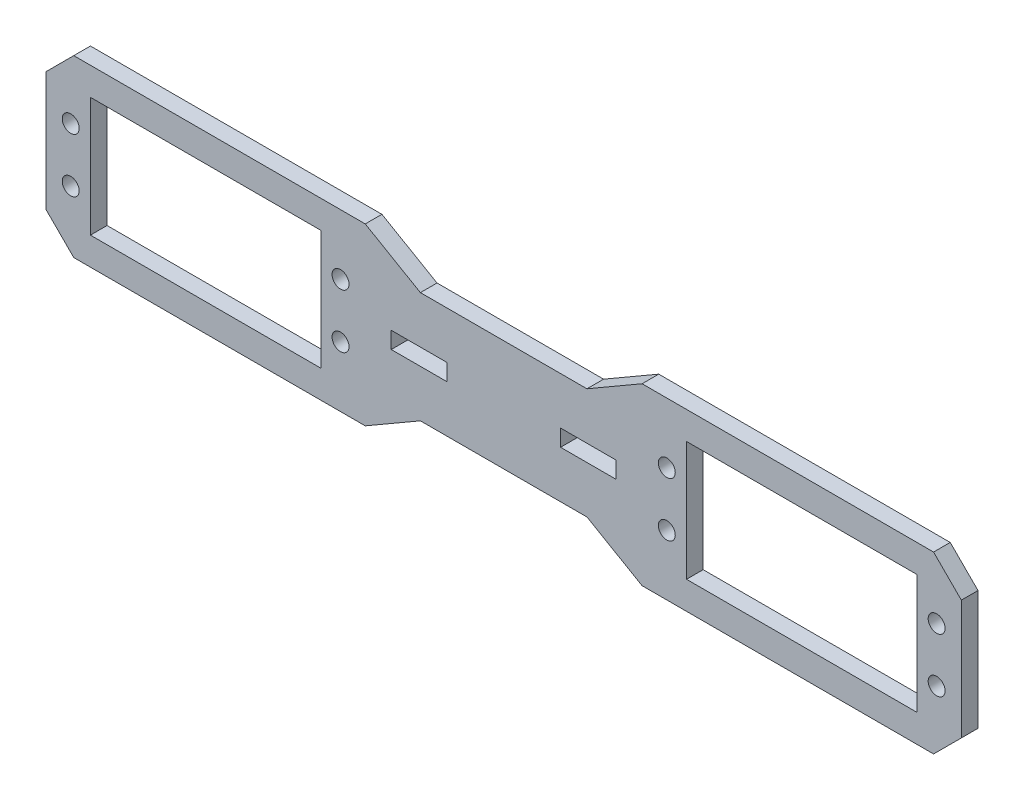
from build123d import *

# Parameters (mm, degrees)
SKETCH_1_R      = 1.525
SKETCH_1_W      = 41.5
SKETCH_1_H      = 21.5
SKETCH_1_W_2    = 10
SKETCH_1_H_2    = 3
EXTRUDE_3_DEPTH = 3


with BuildPart() as part:
    # 草图1 → 凸台-拉伸3 (new body)
    with BuildSketch(Plane.XY):
        Polygon((-77.274452038, 15.659691017), (-82.274452038, 10.659691017), (-82.274452038, -10.840308983), (-77.274452038, -15.840308983), (-24.774452038, -15.840308983), (-14.844452038, -10.090308983), (15.155547962, -10.090308983), (25.085547962, -15.840308983), (77.585547962, -15.840308983), (82.585547962, -10.840308983), (82.585547962, 10.659691017), (77.585547962, 15.659691017), (25.085547962, 15.659691017), (15.155547962, 9.909691017), (-14.844452038, 9.909691017), (-24.774452038, 15.659691017), align=None)
        with Locations((78.135547962, 4.784691017)):
            Circle(SKETCH_1_R, mode=Mode.SUBTRACT)
        with Locations((78.135547962, -4.965308983)):
            Circle(SKETCH_1_R, mode=Mode.SUBTRACT)
        with Locations((-77.824452038, -4.965308983)):
            Circle(SKETCH_1_R, mode=Mode.SUBTRACT)
        with Locations((-77.824452038, 4.784691017)):
            Circle(SKETCH_1_R, mode=Mode.SUBTRACT)
        with Locations((29.535547962, 4.784691017)):
            Circle(SKETCH_1_R, mode=Mode.SUBTRACT)
        with Locations((29.535547962, -4.965308983)):
            Circle(SKETCH_1_R, mode=Mode.SUBTRACT)
        with Locations((-29.224452038, -4.965308983)):
            Circle(SKETCH_1_R, mode=Mode.SUBTRACT)
        with Locations((-29.224452038, 4.784691017)):
            Circle(SKETCH_1_R, mode=Mode.SUBTRACT)
        with Locations((-53.524452038, -0.090308983)):
            Rectangle(SKETCH_1_W, SKETCH_1_H, mode=Mode.SUBTRACT)
        with Locations((53.835547962, -0.090308983)):
            Rectangle(SKETCH_1_W, SKETCH_1_H, mode=Mode.SUBTRACT)
        with Locations((15.403552423, -0.090308983)):
            Rectangle(SKETCH_1_W_2, SKETCH_1_H_2, mode=Mode.SUBTRACT)
        with Locations((-15.092456498, -0.090308983)):
            Rectangle(SKETCH_1_W_2, SKETCH_1_H_2, mode=Mode.SUBTRACT)
    extrude(amount=EXTRUDE_3_DEPTH)


solid = part.part
